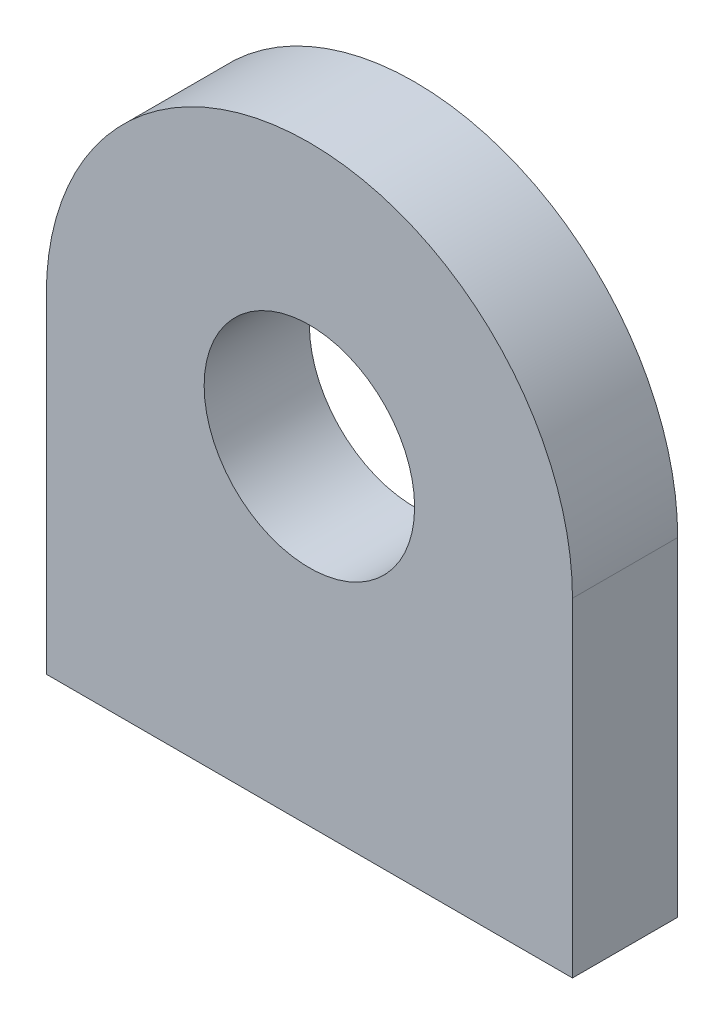
SolidWorks part; units mm, degrees
material "1023 碳钢板 (SS)"
ref_plane "Front Plane" through (0, 0, 0) normal (0, 0, 1) x (1, 0, 0)
ref_plane "Top Plane" through (0, 0, 0) normal (0, 1, 0) x (1, 0, 0)
ref_plane "Right Plane" through (0, 0, 0) normal (1, 0, 0) x (0, 0, -1)
sketch "Sketch1" plane through (0, 0, 0) normal (0, 0, 1) x (1, 0, 0)
  line L0 (-20, 0) -> (-20, -25)
  line L5 (-20, -25) -> (20, -25)
  line L6 (20, -25) -> (20, 0)
  circle A0 centre (0, 0) radius 8
  arc A1 (20, 0) -> (-20, 0) centre (0, 0) ccw
  point P3 (0, -7.9518)
  dimension "D2" = 16
  dimension "D3" = 40
  dimension "D1" = 25
extrude "Boss-Extrude1" add sketch "Sketch1" along normal blind 8 contours A0 | A1 L0 L5 L6
